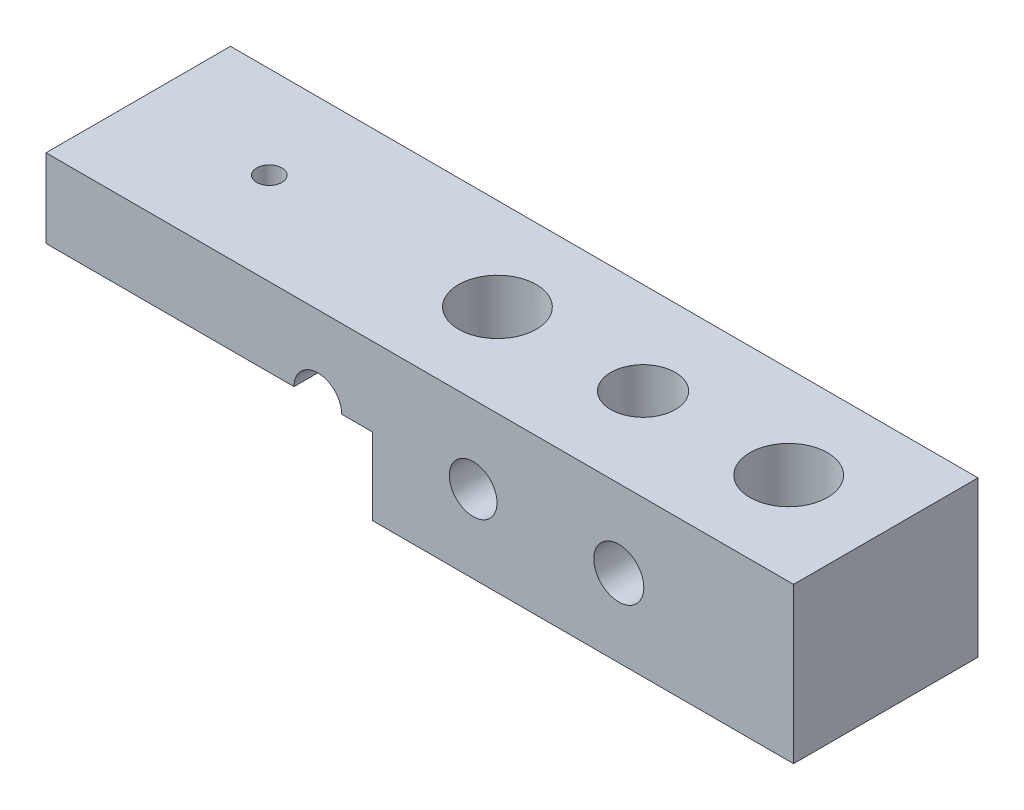
from build123d import *

# Parameters (mm, degrees)
SKETCH1_R           = 2.5765
SKETCH1_R_2         = 2.4585
BOSS_EXTRUDE1_DEPTH = 19
SKETCH2_R           = 4
SKETCH2_R_2         = 3.3235
SKETCH2_R_3         = 1.2995
CUT_EXTRUDE1_DEPTH  = 81.907354425
SKETCH3_R           = 5
CUT_EXTRUDE2_DEPTH  = 5


with BuildPart() as part:
    # Sketch1 → Boss-Extrude1 (new body)
    with BuildSketch(Plane.XY):
        with BuildLine():
            Line((0, 0), (25.5415, 0))
            ThreePointArc((25.5415, 0), (28, 2.4585), (30.4585, 0))
            Line((30.4585, 0), (33.63748457, 0))
            Line((33.63748457, 0), (33.63748457, -7.90741809))
            Line((33.63748457, -7.90741809), (77, -7.90741809))
            Line((77, -7.90741809), (77, 8.09258191))
            Line((77, 8.09258191), (0, 8.09258191))
            Line((0, 8.09258191), (0, 0))
        make_face()
        with Locations((59, 0.09258191)):
            Circle(SKETCH1_R, mode=Mode.SUBTRACT)
        with Locations((44, 0.09258191)):
            Circle(SKETCH1_R_2, mode=Mode.SUBTRACT)
    extrude(amount=BOSS_EXTRUDE1_DEPTH)

    # Sketch2 → Cut-Extrude1 (cut, through all)
    with BuildSketch(Plane(origin=(0, 8.09258191, 0), x_dir=(1, 0, 0), z_dir=(0, 1, 0))):
        with Locations(Location((67, -9.5, 0), (0, 0, 180))):
            Circle(SKETCH2_R)
        with Locations(Location((52, -9.5, 0), (0, 0, 180))):
            Circle(SKETCH2_R_2)
        with Locations(Location((37, -9.5, 0), (0, 0, 180))):
            Circle(SKETCH2_R)
        with Locations(Location((13.50002, -9.5, 0), (0, 0, 180))):
            Circle(SKETCH2_R_3)
    extrude(amount=-CUT_EXTRUDE1_DEPTH, mode=Mode.SUBTRACT)

    # Sketch3 → Cut-Extrude2 (cut)
    with BuildSketch(Plane(origin=(0, 0, 0), x_dir=(-1, 0, 0), z_dir=(0, -1, 0))):
        with Locations(Location((-13.50002, -9.5, 0), (0, 0, 90))):
            Circle(SKETCH3_R)
    extrude(amount=-CUT_EXTRUDE2_DEPTH, mode=Mode.SUBTRACT)


solid = part.part
